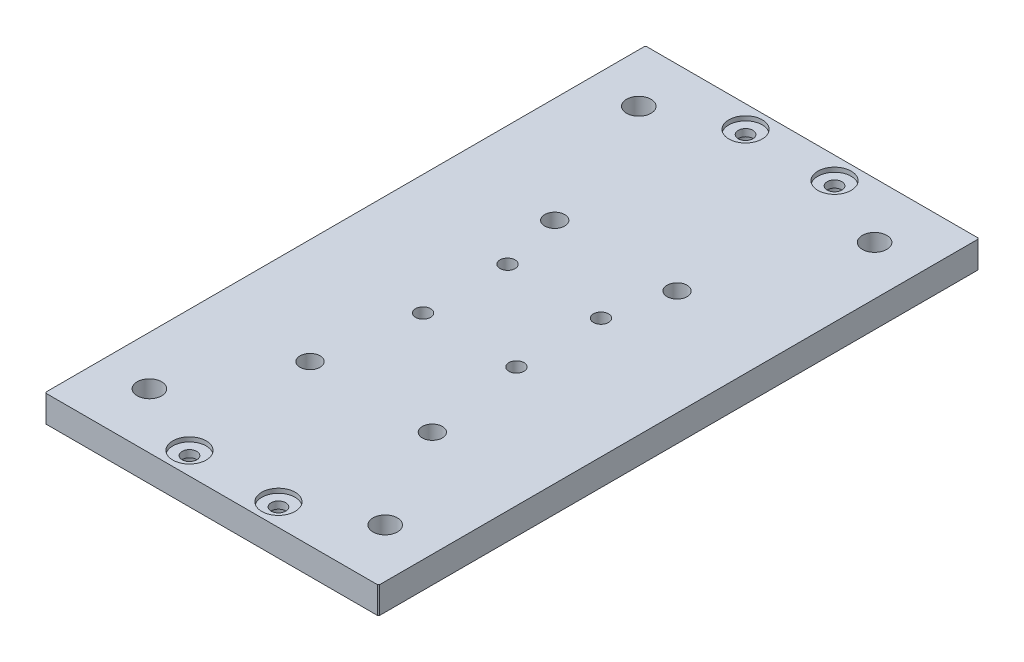
from build123d import *

# Parameters (mm, degrees)
SKETCH1_W                                            = 150
SKETCH1_H                                            = 270
BOSS_EXTRUDE1_DEPTH                                  = 6
SKETCH2_R                                            = 10
CUT_EXTRUDE1_DEPTH                                   = 2
M10_CLEARANCE_HOLE1_D                                = 11
SKETCH5_R                                            = 7.5
CUT_EXTRUDE2_DEPTH                                   = 2
HOLE_SIZE_PER_SOCKET_HEAD_CAP_SCREW_TYPE_D           = 6.6
HOLE_SIZE_PER_SOCKET_HEAD_CAP_SCREW_TYPE_CBORE_D     = 11
HOLE_SIZE_PER_SOCKET_HEAD_CAP_SCREW_TYPE_CBORE_DEPTH = 6.8
M8_TAPPED_HOLE2_D                                    = 6.8
CHAMFER1_SIZE                                        = 0.5
M8_CLEARANCE_HOLE1_D                                 = 9


with BuildPart() as part:
    # Sketch1 → Boss-Extrude1 (new, symmetric)
    with BuildSketch(Plane(origin=(0, 0, 0), x_dir=(1, 0, 0), z_dir=(0, 1, 0))):
        Rectangle(SKETCH1_W, SKETCH1_H)
    extrude(amount=BOSS_EXTRUDE1_DEPTH, both=True)

    # Sketch2 → Cut-Extrude1 (cut)
    with BuildSketch(Plane.XZ.offset(6)):
        with Locations(Location((-53, 110, 0), (0, 0, 270))):
            Circle(SKETCH2_R)
        with Locations(Location((53, 110, 0), (0, 0, 90))):
            Circle(SKETCH2_R)
        with Locations(Location((53, -110, 0), (0, 0, 270))):
            Circle(SKETCH2_R)
        with Locations(Location((-53, -110, 0), (0, 0, 90))):
            Circle(SKETCH2_R)
    extrude(amount=-CUT_EXTRUDE1_DEPTH, mode=Mode.SUBTRACT)

    # M10 Clearance Hole1 (through all)
    with Locations(Plane(origin=(0, 6, 0), x_dir=(1, 0, 0), z_dir=(0, 1, 0))):
        with Locations((-53, 110), (53, 110), (-53, -110), (53, -110)):
            Hole(M10_CLEARANCE_HOLE1_D / 2)

    # Sketch5 → Cut-Extrude2 (cut)
    with BuildSketch(Plane(origin=(0, 6, 0), x_dir=(1, 0, 0), z_dir=(0, 1, 0))):
        with Locations(Location((-20, 125, 0), (0, 0, 270))):
            Circle(SKETCH5_R)
        with Locations(Location((20, 125, 0), (0, 0, 90))):
            Circle(SKETCH5_R)
        with Locations(Location((20, -125, 0), (0, 0, 270))):
            Circle(SKETCH5_R)
        with Locations(Location((-20, -125, 0), (0, 0, 90))):
            Circle(SKETCH5_R)
    extrude(amount=-CUT_EXTRUDE2_DEPTH, mode=Mode.SUBTRACT)

    # Hole size per socket head cap screw type 1 (through all)
    with Locations(Plane(origin=(0, -6, 0), x_dir=(-1, 0, 0), z_dir=(0, -1, 0))):
        with Locations((20, -125), (-20, -125), (20, 125), (-20, 125)):
            CounterBoreHole(HOLE_SIZE_PER_SOCKET_HEAD_CAP_SCREW_TYPE_D / 2, HOLE_SIZE_PER_SOCKET_HEAD_CAP_SCREW_TYPE_CBORE_D / 2, HOLE_SIZE_PER_SOCKET_HEAD_CAP_SCREW_TYPE_CBORE_DEPTH)

    # M8 Tapped Hole2 (through all)
    with Locations(Plane(origin=(0, -6, 0), x_dir=(-1, 0, 0), z_dir=(0, -1, 0))):
        with Locations((21, 19), (21, -19), (-21, -19), (-21, 19)):
            Hole(M8_TAPPED_HOLE2_D / 2)

    # Chamfer1
    chamfer1_edges = [part.edges().sort_by_distance(p)[0] for p in [
        (75, 0, 135),
        (-75, 0, 135),
        (-75, 0, -135),
        (75, 0, -135),
    ]]
    chamfer(chamfer1_edges, length=CHAMFER1_SIZE)

    # M8 Clearance Hole1 (through all)
    with Locations(Plane(origin=(0, 6, 0), x_dir=(1, 0, 0), z_dir=(0, 1, 0))):
        with Locations((27.5, 46.7), (-27.5, 46.7), (27.5, -63.3), (-27.5, -63.3)):
            Hole(M8_CLEARANCE_HOLE1_D / 2)


solid = part.part
